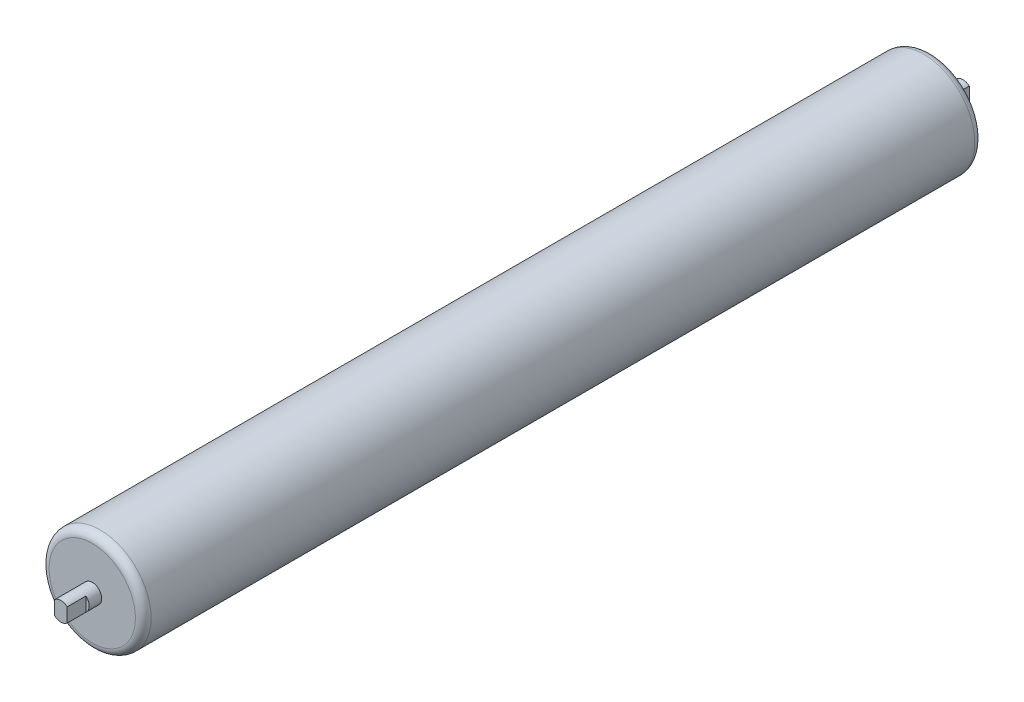
SolidWorks part; units mm, degrees
ref_plane "前视基准面" through (0, 0, 0) normal (0, 0, 1) x (1, 0, 0)
ref_plane "上视基准面" through (0, 0, 0) normal (0, 1, 0) x (1, 0, 0)
ref_plane "右视基准面" through (0, 0, 0) normal (1, 0, 0) x (0, 0, -1)
sketch "草图1" plane through (0, 0, 0) normal (0, 0, 1) x (1, 0, 0)
  circle A0 centre (0, 0) radius 32.5
  dimension "D1" = 65
extrude "凸台-拉伸1" add sketch "草图1" along normal mid plane 535
sketch "草图2" plane through (0, 0, -267.5) normal (0, 0, -1) x (-1, 0, 0)
  circle A0 centre (0, 0) radius 6
  dimension "D1" = 12
extrude "凸台-拉伸2" add sketch "草图2" along normal blind 20
sketch "草图3" plane through (0, 0, -287.5) normal (0, 0, -1) x (-1, 0, 0)
  line L1 (-4, 6.4215) -> (4, 6.4215)
  line L2 (-4, 6.4215) -> (-4, -6.4215)
  line L3 (-4, -6.4215) -> (4, -6.4215)
  line L4 (4, 6.4215) -> (4, -6.4215)
  line L5 (-4, 6.4215) -> (4, -6.4215) construction
  line L6 (-4, -6.4215) -> (4, 6.4215) construction
  point P0 (0, 0)
  dimension "D1" = 8
extrude "切除-拉伸1" cut sketch "草图3" against normal blind 12 flip side to cut
mirror "镜向1" about plane through (0, 0, 0) normal (0, 0, 1) of "切除-拉伸1", "凸台-拉伸2"
fillet "圆角1" radius 5 2 edges at (32.5, 0, 267.5) (32.5, 0, -267.5)
